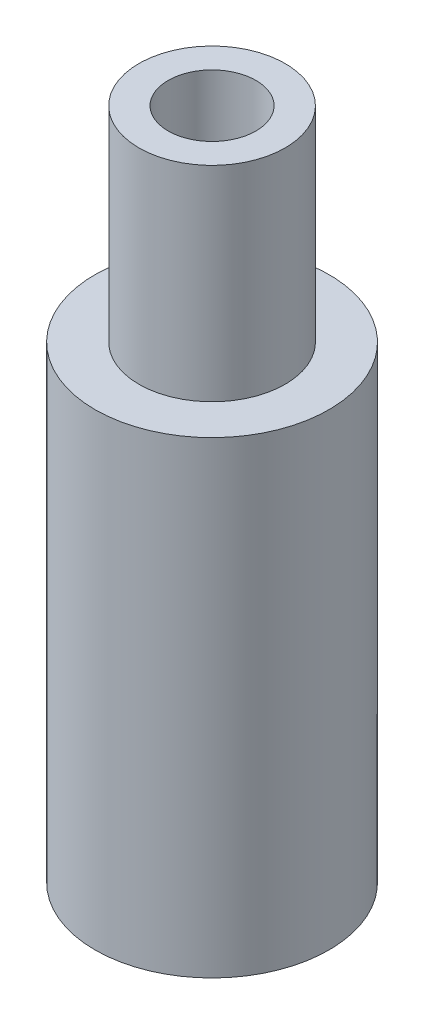
from build123d import *


with BuildPart() as part:
    # Sketch1 → Revolve1 (revolve)
    with BuildSketch(Plane.XY, mode=Mode.PRIVATE) as revolve1_sk:
        Polygon((-65.629373749, -27.972671928), (-60.629373749, -27.972671928), (-60.629373749, -62.972671928), (-53.129373749, -62.972671928), (-53.129373749, -142.972671928), (-73.129373749, -142.972671928), (-73.129373749, -137.972671928), (-58.129373749, -137.972671928), (-58.129373749, -67.972671928), (-65.629373749, -67.972671928), align=None)
    revolve(revolve1_sk.sketch.rotate(Axis((-73.129373749, -60, 0), (0, -1, 0)), 90), axis=Axis((-73.129373749, -60, 0), (0, -1, 0)))


solid = part.part
